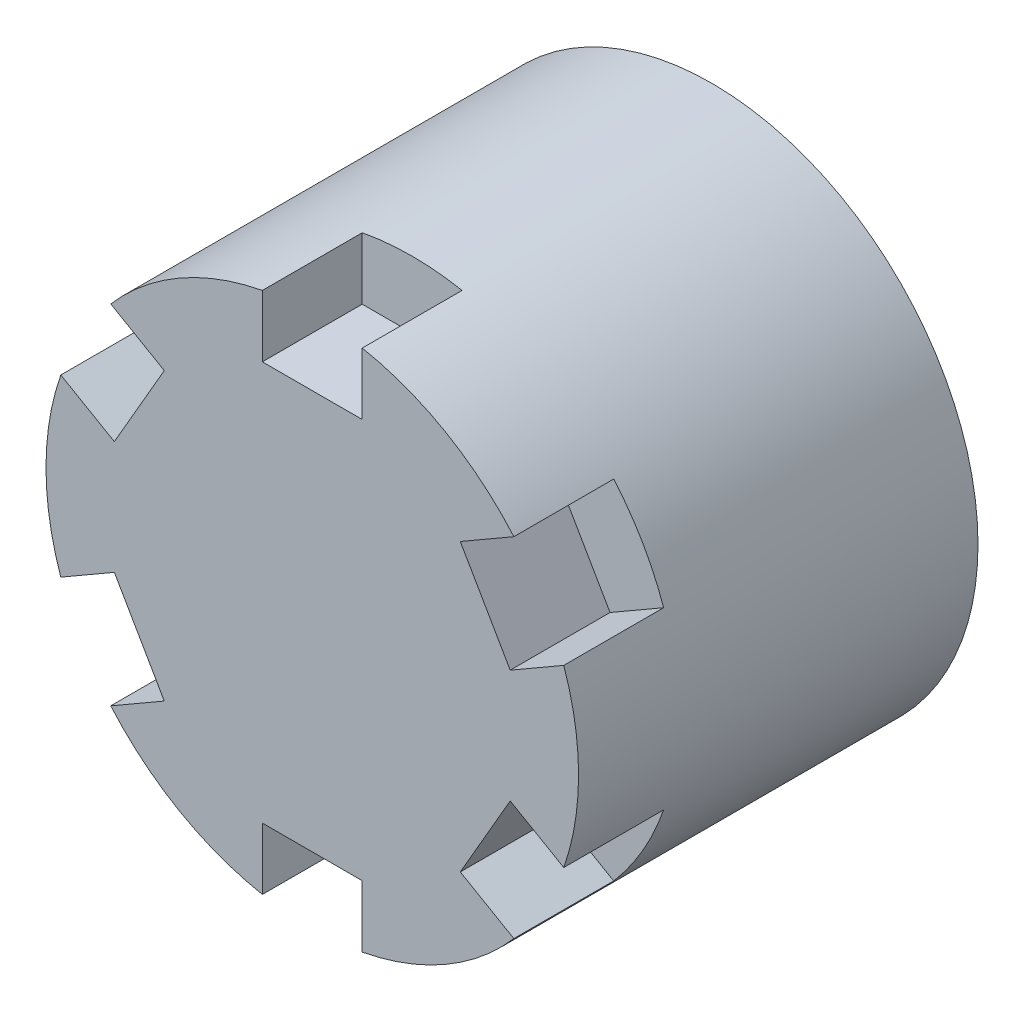
SolidWorks part; units mm, degrees
ref_plane "前视基准面" through (0, 0, 0) normal (0, 0, 1) x (1, 0, 0)
ref_plane "上视基准面" through (0, 0, 0) normal (0, 1, 0) x (1, 0, 0)
ref_plane "右视基准面" through (0, 0, 0) normal (1, 0, 0) x (0, 0, -1)
other "Configuration Table"
sketch "草图1" plane through (0, 0, 0) normal (0, 0, 1) x (1, 0, 0)
  circle A0 centre (0, 0) radius 19.5
  dimension "D1" = 39
sketch "草图2" plane through (0, 0, 0) normal (0, 0, 1) x (1, 0, 0)
  circle A0 centre (0, 0) radius 40
  dimension "D1" = 80
extrude "凸台-拉伸1" add sketch "草图2" along normal blind 60 contours A0
extrude "切除-拉伸1" cut sketch "草图1" along normal blind 40 contours A0
sketch "草图3" plane through (0, 0, 60) normal (0, 0, 1) x (1, 0, 0)
  line L0 (22.2308, 21.4952) -> (29.7308, 8.5048)
  line L2 (-7.5, 39.2906) -> (-7.5, 30)
  line L3 (-7.5, 30) -> (7.5, 30)
  line L4 (7.5, 39.2906) -> (7.5, 30)
  line L5 (37.7766, 13.1501) -> (29.7308, 8.5048)
  line L6 (30.2766, 26.1405) -> (22.2308, 21.4952)
  line L7 (29.7308, -8.5048) -> (22.2308, -21.4952)
  line L8 (30.2766, -26.1405) -> (22.2308, -21.4952)
  line L9 (37.7766, -13.1501) -> (29.7308, -8.5048)
  line L10 (7.5, -30) -> (-7.5, -30)
  line L11 (-7.5, -39.2906) -> (-7.5, -30)
  line L12 (7.5, -39.2906) -> (7.5, -30)
  line L13 (-22.2308, -21.4952) -> (-29.7308, -8.5048)
  line L14 (-37.7766, -13.1501) -> (-29.7308, -8.5048)
  line L15 (-30.2766, -26.1405) -> (-22.2308, -21.4952)
  line L16 (-29.7308, 8.5048) -> (-22.2308, 21.4952)
  line L17 (-30.2766, 26.1405) -> (-22.2308, 21.4952)
  line L18 (-37.7766, 13.1501) -> (-29.7308, 8.5048)
  circle A0 centre (0, 0) radius 40 construction
  arc A1 (7.5, 39.2906) -> (-7.5, 39.2906) centre (0, 0) ccw
  arc A2 (37.7766, 13.1501) -> (30.2766, 26.1405) centre (0, 0) ccw
  arc A3 (30.2766, -26.1405) -> (37.7766, -13.1501) centre (0, 0) ccw
  arc A4 (-7.5, -39.2906) -> (7.5, -39.2906) centre (0, 0) ccw
  arc A5 (-37.7766, -13.1501) -> (-30.2766, -26.1405) centre (0, 0) ccw
  arc A6 (-30.2766, 26.1405) -> (-37.7766, 13.1501) centre (0, 0) ccw
  point P7 (0, 30)
  dimension "D1" = 15
  dimension "D2" = 30
  dimension "D3" = 6
extrude "切除-拉伸2" cut sketch "草图3" against normal blind 15
sketch "草图4" plane through (0, 0, 0) normal (0, 0, -1) x (-1, 0, 0)
  line L1 (-10, 23) -> (10, 23)
  line L2 (-10, 23) -> (-10, 15.9176)
  line L3 (-10, 15.9176) -> (10, 15.9176)
  line L4 (10, 23) -> (10, 15.9176)
  point P4 (0, 15.9176)
  dimension "D1" = 20
  dimension "D2" = 23
extrude "切除-拉伸3" cut sketch "草图4" against normal blind 30 contours L4 L3 L2 L1
